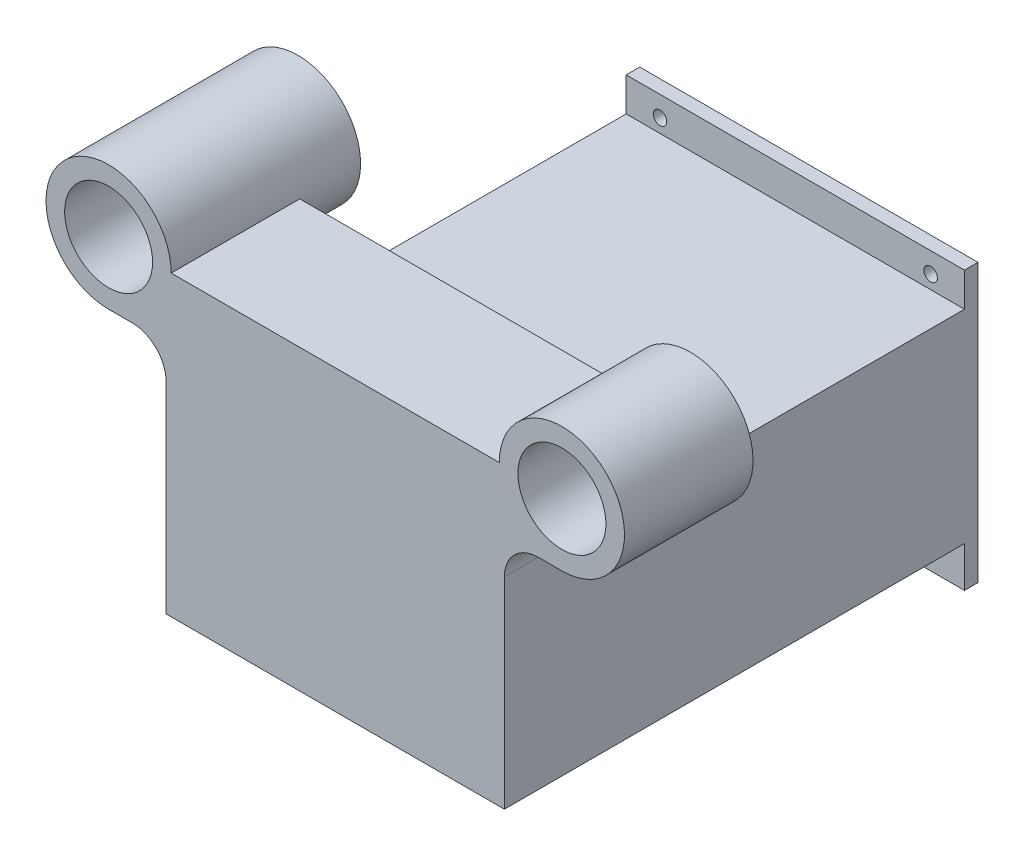
from build123d import *
from build123d.topology import SkipClean

# Parameters (mm, degrees)
SKETCH_2_R          = 13
EXTRUDE_1_DEPTH     = 38
SKETCH_23_W         = 100
SKETCH_23_H         = 60
SKETCH_23_W_2       = 92
SKETCH_23_H_2       = 42
EXTRUDE_7_DEPTH     = 102
SKETCH_25_R         = 7
CUT_EXTRUDE_4_DEPTH = 50
EXTRUDE_START       = 18
SKETCH_26_R         = 18.5
SKETCH_26_R_2       = 13
EXTRUDE_8_DEPTH     = 18
SKETCH_28_W         = 92
SKETCH_28_H         = 42
CUT_EXTRUDE_5_DEPTH = 30
SKETCH_29_W         = 92
SKETCH_29_H         = 67
EXTRUDE_9_DEPTH     = 4
SKETCH_32_W         = 100
SKETCH_32_H         = 10
SKETCH_32_H_2       = 12
EXTRUDE_10_DEPTH    = 4
SKETCH_33_R         = 2
CUT_EXTRUDE_6_DEPTH = 4


with BuildPart() as part:
    # 草图2 → 凸台-拉伸1 (new body)
    with BuildSketch(Plane.XY):
        with BuildLine():
            Line((-48.5, 0), (48.5, 0))
            ThreePointArc((48.5, 0), (80.081475452, 13.081475452), (67, -18.5))
            Line((67, -18.5), (60, -18.5))
            ThreePointArc((60, -18.5), (52.928932188, -21.428932188), (50, -28.5))
            Line((50, -28.5), (50, -88))
            Line((50, -88), (-50, -88))
            Line((-50, -88), (-50, -28.5))
            ThreePointArc((-50, -28.5), (-52.928932188, -21.428932188), (-60, -18.5))
            Line((-60, -18.5), (-67, -18.5))
            ThreePointArc((-67, -18.5), (-80.081475452, 13.081475452), (-48.5, 0))
        make_face()
        with Locations((-67, 0)):
            Circle(SKETCH_2_R, mode=Mode.SUBTRACT)
        with Locations(Location((67, 0, 0), (0, 0, 180))):
            Circle(SKETCH_2_R, mode=Mode.SUBTRACT)
    extrude(amount=EXTRUDE_1_DEPTH)

    # 草图23 → 凸台-拉伸7 (add)
    with BuildSketch(Plane(origin=(0, 0, 0), x_dir=(-1, 0, 0), z_dir=(0, 0, -1))):
        with Locations((0, -58)):
            Rectangle(SKETCH_23_W, SKETCH_23_H)
        with Locations((0, -57)):
            Rectangle(SKETCH_23_W_2, SKETCH_23_H_2, mode=Mode.SUBTRACT)
    extrude(amount=EXTRUDE_7_DEPTH)

    # 草图25 → 切除-拉伸4 (cut)
    with BuildSketch(Plane(origin=(0, -88, 0), x_dir=(-1, 0, 0), z_dir=(0, -1, 0))):
        with Locations(Location((0, 14, 0), (0, 0, 90))):
            Circle(SKETCH_25_R)
    extrude(amount=-CUT_EXTRUDE_4_DEPTH, mode=Mode.SUBTRACT)

    # 草图26 → 凸台-拉伸8 (add)
    with SkipClean():  # the faces are left unmerged after this step: merging them gives an invalid solid
        with BuildSketch(Plane(origin=(0, 0, 0), x_dir=(-1, 0, 0), z_dir=(0, 0, -1)).offset(EXTRUDE_START)):
            with Locations((67, 0)):
                Circle(SKETCH_26_R)
            with Locations((67, 0)):
                Circle(SKETCH_26_R_2, mode=Mode.SUBTRACT)
        extrude(amount=-EXTRUDE_8_DEPTH)

    # 草图28 → 切除-拉伸5 (cut)
    with SkipClean():  # the faces are left unmerged after this step: merging them gives an invalid solid
        with BuildSketch(Plane(origin=(0, 0, 0), x_dir=(-1, 0, 0), z_dir=(0, 0, -1))):
            with Locations((0, -57)):
                Rectangle(SKETCH_28_W, SKETCH_28_H)
        extrude(amount=-CUT_EXTRUDE_5_DEPTH, mode=Mode.SUBTRACT)

    # 草图29 → 凸台-拉伸9 (add)
    with SkipClean():  # the faces are left unmerged after this step: merging them gives an invalid solid
        with BuildSketch(Plane(origin=(0, -36, 0), x_dir=(-1, 0, 0), z_dir=(0, -1, 0))):
            with Locations((0, 3.48412197)):
                Rectangle(SKETCH_29_W, SKETCH_29_H)
        extrude(amount=EXTRUDE_9_DEPTH)

    # 草图30 → 切除-旋转3 (revolve, cut)
    with SkipClean():  # the faces are left unmerged after this step: merging them gives an invalid solid
        with BuildSketch(Plane.XY.offset(-14), mode=Mode.PRIVATE) as cut_revolve_3_sk:
            Polygon((0, -88), (-8, -88), (-8, -85.4), (-12, -85.4), (-12, -84.256), (-14, -84.256), (-14, -36.11445811), (-7.5, -36.11445811), (-7.5, -35), (-7, -35), (-7, -31.9), (0, -31.9), align=None)
        revolve(cut_revolve_3_sk.sketch.rotate(Axis((0, -88, -14), (0, 1, 0)), 180), axis=Axis((0, -88, -14), (0, 1, 0)), mode=Mode.SUBTRACT)

    # 草图31 → 切除-旋转4 (revolve, cut)
    with SkipClean():  # the faces are left unmerged after this step: merging them gives an invalid solid
        with BuildSketch(Plane.XY.offset(-59.8), mode=Mode.PRIVATE) as cut_revolve_4_sk:
            Polygon((0, -84.7), (-6.7, -84.7), (-6.7, -82.7), (-7.5, -82.7), (-7.5, -30.816), (-6.7, -30.816), (-6.7, -28.816), (0, -28.816), align=None)
        revolve(cut_revolve_4_sk.sketch.rotate(Axis((0, -84.7, -59.8), (0, 1, 0)), 180), axis=Axis((0, -84.7, -59.8), (0, 1, 0)), mode=Mode.SUBTRACT)

    # 草图32 → 凸台-拉伸10 (add)
    with SkipClean():  # the faces are left unmerged after this step: merging them gives an invalid solid
        with BuildSketch(Plane(origin=(0, 0, -102), x_dir=(-1, 0, 0), z_dir=(0, 0, -1))):
            with Locations((0, -23)):
                Rectangle(SKETCH_32_W, SKETCH_32_H)
            with Locations((0, -94)):
                Rectangle(SKETCH_32_W, SKETCH_32_H_2)
        extrude(amount=-EXTRUDE_10_DEPTH)

    # 草图33 → 切除-拉伸6 (cut)
    with SkipClean():  # the faces are left unmerged after this step: merging them gives an invalid solid
        with BuildSketch(Plane(origin=(0, 0, -102), x_dir=(-1, 0, 0), z_dir=(0, 0, -1))):
            with Locations((-40, -94.057478358)):
                Circle(SKETCH_33_R)
            with Locations((-40, -24)):
                Circle(SKETCH_33_R)
            with Locations(Location((40, -94.057478358, 0), (0, 0, 180))):
                Circle(SKETCH_33_R)
            with Locations(Location((40, -24, 0), (0, 0, 180))):
                Circle(SKETCH_33_R)
        extrude(amount=-CUT_EXTRUDE_6_DEPTH, mode=Mode.SUBTRACT)


solid = part.part
